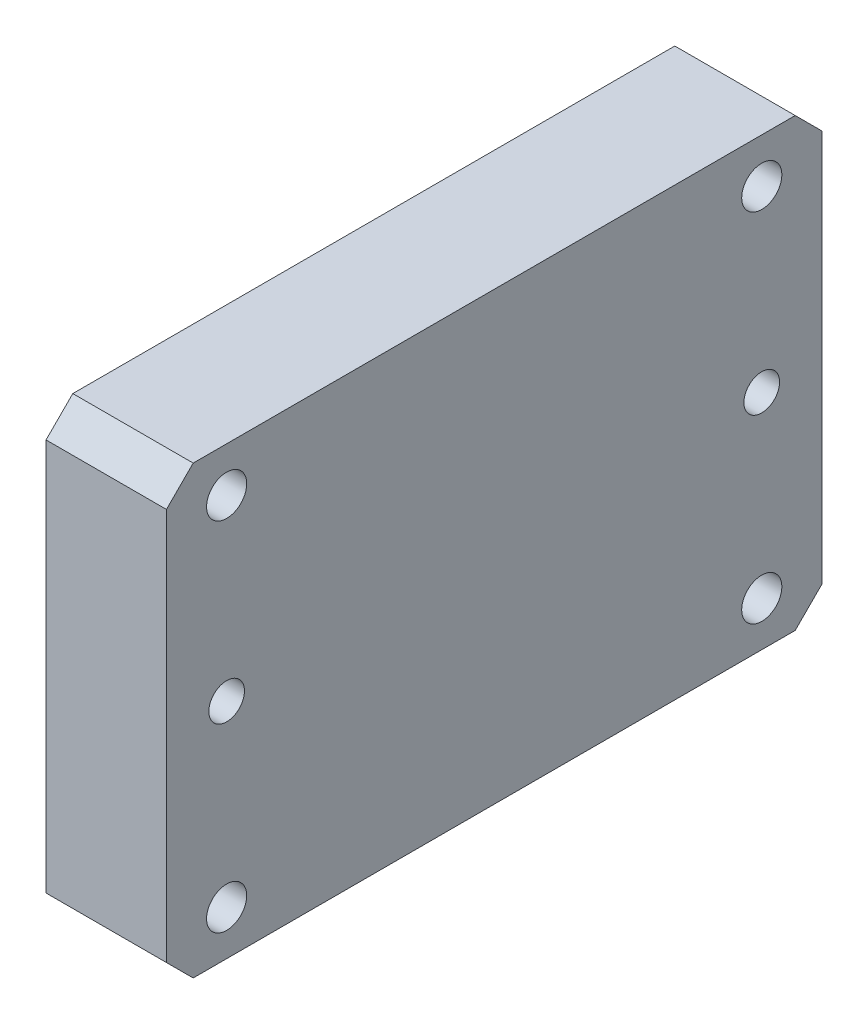
from build123d import *

# Parameters (mm, degrees)
SKETCH1_W                                            = 73.5
SKETCH1_H                                            = 50
BOSS_EXTRUDE1_DEPTH                                  = 13.5
CBORE_FOR_M4_HEXAGON_SOCKET_HEAD_CAP_SCR_D           = 4.5
CBORE_FOR_M4_HEXAGON_SOCKET_HEAD_CAP_SCR_CBORE_D     = 8
CBORE_FOR_M4_HEXAGON_SOCKET_HEAD_CAP_SCR_CBORE_DEPTH = 4.6
F_4_0MM_DOWEL_HOLE1_D                                = 4
F_4_0MM_DOWEL_HOLE1_DEPTH                            = 6
F_4_0MM_DOWEL_HOLE1_TIP                              = 1.201721238
M4_TAPPED_HOLE1_D                                    = 3.3
M4_TAPPED_HOLE1_DEPTH                                = 10.1
M4_TAPPED_HOLE1_TIP                                  = 0.991420021
CHAMFER1_SIZE                                        = 3


with BuildPart() as part:
    # Sketch1 → Boss-Extrude1 (new body)
    with BuildSketch(Plane(origin=(0, 0, 0), x_dir=(0, 0, -1), z_dir=(1, 0, 0))):
        Rectangle(SKETCH1_W, SKETCH1_H)
    extrude(amount=BOSS_EXTRUDE1_DEPTH)

    # CBORE for M4 Hexagon socket head cap screws1 (through all)
    with Locations(Plane.ZY):
        with Locations((30, -20), (30, 20), (-30, 20), (-30, -20)):
            CounterBoreHole(CBORE_FOR_M4_HEXAGON_SOCKET_HEAD_CAP_SCR_D / 2, CBORE_FOR_M4_HEXAGON_SOCKET_HEAD_CAP_SCR_CBORE_D / 2, CBORE_FOR_M4_HEXAGON_SOCKET_HEAD_CAP_SCR_CBORE_DEPTH)

    # Ø4.0mm Dowel Hole1
    with Locations(Plane(origin=(13.5, 0, 0), x_dir=(0, 0, -1), z_dir=(1, 0, 0))):
        with Locations((30, 0), (-30, 0)):
            Hole(F_4_0MM_DOWEL_HOLE1_D / 2, depth=F_4_0MM_DOWEL_HOLE1_DEPTH)
            with Locations((0, 0, -(F_4_0MM_DOWEL_HOLE1_DEPTH + F_4_0MM_DOWEL_HOLE1_TIP / 2))):  # 118° drill point
                Cone(0, F_4_0MM_DOWEL_HOLE1_D / 2, F_4_0MM_DOWEL_HOLE1_TIP, mode=Mode.SUBTRACT)

    # M4 Tapped Hole1
    with Locations(Plane.ZY):
        with Locations((28.25, -11.25), (-30.75, -11.25)):
            Hole(M4_TAPPED_HOLE1_D / 2, depth=M4_TAPPED_HOLE1_DEPTH)
            with Locations((0, 0, -(M4_TAPPED_HOLE1_DEPTH + M4_TAPPED_HOLE1_TIP / 2))):  # 118° drill point
                Cone(0, M4_TAPPED_HOLE1_D / 2, M4_TAPPED_HOLE1_TIP, mode=Mode.SUBTRACT)

    # Chamfer1
    chamfer1_edges = [part.edges().sort_by_distance(p)[0] for p in [
        (6.75, -25, -36.75),
        (6.75, -25, 36.75),
        (6.75, 25, 36.75),
        (6.75, 25, -36.75),
    ]]
    chamfer(chamfer1_edges, length=CHAMFER1_SIZE)


solid = part.part
